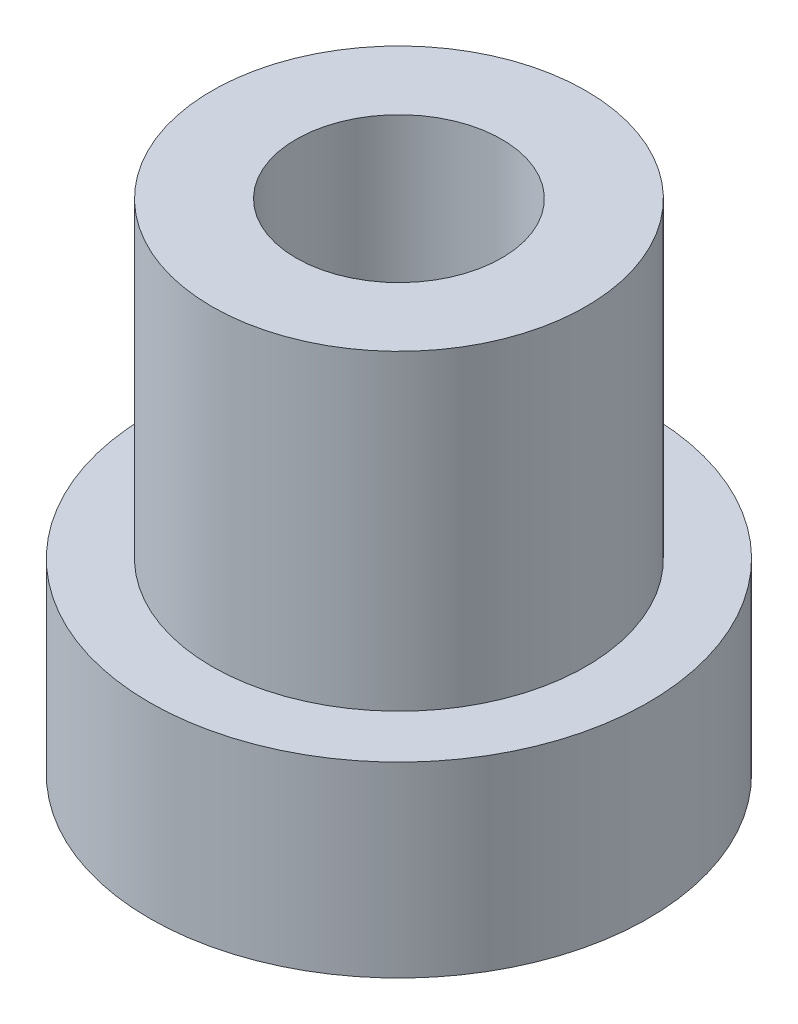
SolidWorks part; units mm, degrees
ref_plane "Front Plane" through (0, 0, 0) normal (0, 0, 1) x (1, 0, 0)
ref_plane "Top Plane" through (0, 0, 0) normal (0, 1, 0) x (1, 0, 0)
ref_plane "Right Plane" through (0, 0, 0) normal (1, 0, 0) x (0, 0, -1)
sketch "Sketch1" plane through (0, 0, 0) normal (0, 0, 1) x (1, 0, 0)
  line L0 (3, 0) -> (3, -5)
  line L1 (0, 0) -> (3, 0)
  line L3 (0, -8) -> (4, -8)
  line L4 (4, -5) -> (4, -8)
  line L5 (3, -5) -> (4, -5)
  line L6 (0, 0) -> (0, -8)
  line L7 (0, 0) -> (0, -9.7456) construction
  dimension "D1" = 4
  dimension "D2" = 3
  dimension "D3" = 3
  dimension "D5" = 8
revolve "Revolve1" add sketch "Sketch1" angle 360 about L6
sketch "Sketch2" plane through (0, 0, 0) normal (0, 1, 0) x (1, 0, 0)
  point P0 (0, 0)
hole_wizard "M4 Tapped Hole1" positions "3DSketch1" profile "Sketch3" tap size "M4" standard "GB" end condition up to next
sketch3d "3DSketch1"
  point P3 (0, 0, 0)
sketch "Sketch3" plane through (0, 0, 0) normal (1, 0, 0) x (0, 0, 1)
  line L0 (0, 0) -> (0, 8)
  line L1 (0, 8) -> (1.65, 8)
  line L2 (1.65, 8) -> (1.65, 0)
  line L5 (1.65, 0) -> (0, 0)
  line L11 (0, -6.35) -> (0, 107.95) construction
  dimension "通孔螺纹孔钻头直径" = 3.3
  dimension "通孔螺纹孔钻头深度" = 8
cosmetic thread "Cosmetic Thread3"
